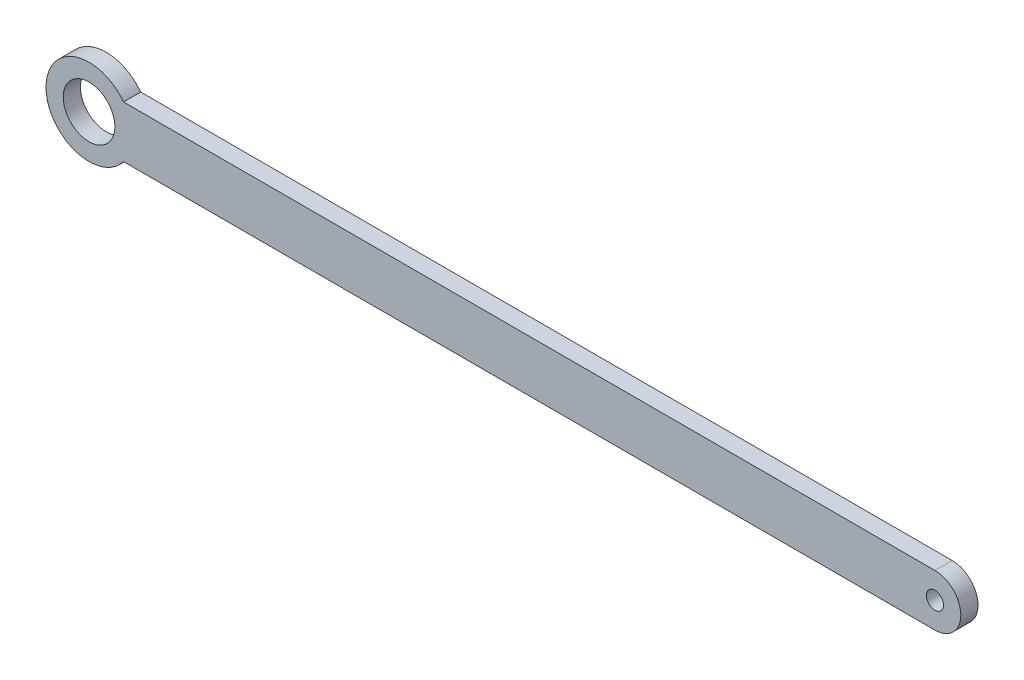
SolidWorks part; units mm, degrees
ref_plane "Front plane" through (0, 0, 0) normal (0, 0, 1) x (1, 0, 0)
ref_plane "Top plane" through (0, 0, 0) normal (0, 1, 0) x (1, 0, 0)
ref_plane "Right plane" through (0, 0, 0) normal (1, 0, 0) x (0, 0, -1)
sketch "Sketch 2" plane through (0, 0, 0) normal (0, 0, 1) x (1, 0, 0)
  line L0 (0, 0) -> (49.128, 0) construction
  line L1 (49.128, 1.5) -> (2, 1.5)
  line L3 (2, -1.5) -> (49.128, -1.5)
  circle A0 centre (0, 0) radius 1.5
  arc A1 (2, 1.5) -> (2, -1.5) centre (0, 0) ccw
  circle A2 centre (49.128, 0) radius 0.5
  arc A3 (49.128, -1.5) -> (49.128, 1.5) centre (49.128, 0) ccw
  dimension "D1" = 3
  dimension "D2" = 5
  dimension "D3" = 1
  dimension "D4" = 1.5
  dimension "D6" = 49.128
extrude "Boss-Extrude 1" add sketch "Sketch 2" along normal blind 1
